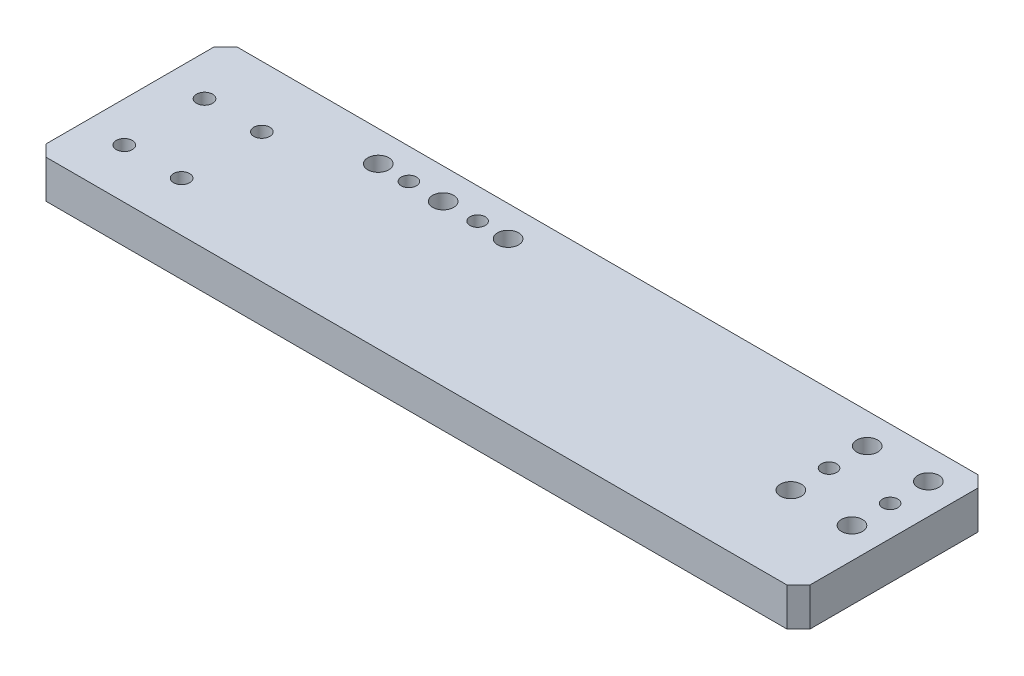
from build123d import *

# Parameters (mm, degrees)
SKETCH_6_W                  = 200
SKETCH_6_H                  = 50
EXTRUDE_1_DEPTH             = 10
CHAMFER_1_SIZE              = 3
HOLE_WIZARD_5_5_5_5_1_D     = 5.5
HOLE_WIZARD_5_5_5_5_1_DEPTH = 12.4
HOLE_WIZARD_5_5_5_5_1_TIP   = 1.652366702
MM_2_D                      = 4
MM_2_DEPTH                  = 12.4
MM_2_TIP                    = 1.201721238
HOLE_WIZARD_M5_2_D          = 4.2
HOLE_WIZARD_M5_2_DEPTH      = 12.4
HOLE_WIZARD_M5_2_TIP        = 1.2618073
HOLE_WIZARD_5_5_5_5_2_D     = 5.5
HOLE_WIZARD_5_5_5_5_2_DEPTH = 12.4
HOLE_WIZARD_5_5_5_5_2_TIP   = 1.652366702
MM_3_D                      = 4
MM_3_DEPTH                  = 12.4
MM_3_TIP                    = 1.201721238


with BuildPart() as part:
    # 草图6 → 凸台-拉伸1 (new body)
    with BuildSketch(Plane(origin=(0, 0, 0), x_dir=(1, 0, 0), z_dir=(0, 1, 0))):
        Rectangle(SKETCH_6_W, SKETCH_6_H)
    extrude(amount=EXTRUDE_1_DEPTH)

    # 倒角1
    chamfer_1_edges = [part.edges().sort_by_distance(p)[0] for p in [
        (100, 5, 25),
        (-100, 5, 25),
        (-100, 5, -25),
        (100, 5, -25),
    ]]
    chamfer(chamfer_1_edges, length=CHAMFER_1_SIZE)

    # Ø5.5 (5.5) 直径孔1
    with Locations(Plane(origin=(0, 10, 0), x_dir=(1, 0, 0), z_dir=(0, 1, 0))):
        with Locations((76, 17), (76, -3), (92, -3), (92, 17)):
            Hole(HOLE_WIZARD_5_5_5_5_1_D / 2, depth=HOLE_WIZARD_5_5_5_5_1_DEPTH)
            with Locations((0, 0, -(HOLE_WIZARD_5_5_5_5_1_DEPTH + HOLE_WIZARD_5_5_5_5_1_TIP / 2))):  # 118° drill point
                Cone(0, HOLE_WIZARD_5_5_5_5_1_D / 2, HOLE_WIZARD_5_5_5_5_1_TIP, mode=Mode.SUBTRACT)

    # 大小mm 暗销孔2
    with Locations(Plane(origin=(0, 10, 0), x_dir=(1, 0, 0), z_dir=(0, 1, 0))):
        with Locations((76, 7), (92, 7)):
            Hole(MM_2_D / 2, depth=MM_2_DEPTH)
            with Locations((0, 0, -(MM_2_DEPTH + MM_2_TIP / 2))):  # 118° drill point
                Cone(0, MM_2_D / 2, MM_2_TIP, mode=Mode.SUBTRACT)

    # M5 螺纹孔2
    with Locations(Plane(origin=(0, 10, 0), x_dir=(1, 0, 0), z_dir=(0, 1, 0))):
        with Locations((-89.5, 9), (-74.5, 9), (-89.5, -12), (-74.5, -12)):
            Hole(HOLE_WIZARD_M5_2_D / 2, depth=HOLE_WIZARD_M5_2_DEPTH)
            with Locations((0, 0, -(HOLE_WIZARD_M5_2_DEPTH + HOLE_WIZARD_M5_2_TIP / 2))):  # 118° drill point
                Cone(0, HOLE_WIZARD_M5_2_D / 2, HOLE_WIZARD_M5_2_TIP, mode=Mode.SUBTRACT)

    # Ø5.5 (5.5) 直径孔2
    with Locations(Plane(origin=(0, 0, 0), x_dir=(-1, 0, 0), z_dir=(0, -1, 0))):
        with Locations((52, 17), (35, 16.974257895), (18, 16.974257895)):
            Hole(HOLE_WIZARD_5_5_5_5_2_D / 2, depth=HOLE_WIZARD_5_5_5_5_2_DEPTH)
            with Locations((0, 0, -(HOLE_WIZARD_5_5_5_5_2_DEPTH + HOLE_WIZARD_5_5_5_5_2_TIP / 2))):  # 118° drill point
                Cone(0, HOLE_WIZARD_5_5_5_5_2_D / 2, HOLE_WIZARD_5_5_5_5_2_TIP, mode=Mode.SUBTRACT)

    # 大小mm 暗销孔3
    with Locations(Plane(origin=(0, 0, 0), x_dir=(-1, 0, 0), z_dir=(0, -1, 0))):
        with Locations((44, 17), (26, 17)):
            Hole(MM_3_D / 2, depth=MM_3_DEPTH)
            with Locations((0, 0, -(MM_3_DEPTH + MM_3_TIP / 2))):  # 118° drill point
                Cone(0, MM_3_D / 2, MM_3_TIP, mode=Mode.SUBTRACT)


solid = part.part
